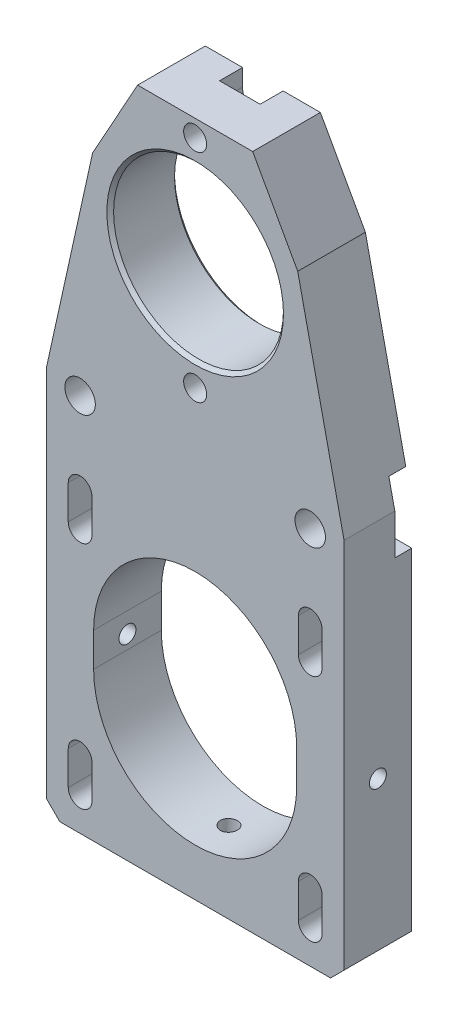
from build123d import *

# Parameters (mm, degrees)
SKETCH1_W                                            = 44
SKETCH1_H                                            = 100
BOSS_EXTRUDE1_DEPTH                                  = 10
SKETCH2_R                                            = 12.55
CUT_EXTRUDE1_DEPTH                                   = 56.533773508
CUT_EXTRUDE3_DEPTH                                   = 56.533773508
CUT_EXTRUDE12_DEPTH                                  = 4.6
LPATTERN1_COUNT                                      = 2
LPATTERN1_PITCH                                      = 34
LPATTERN1_COUNT_DIR2                                 = 2
LPATTERN1_PITCH_DIR2                                 = 34
CHAMFER1_SIZE                                        = 2
CUT_EXTRUDE10_DEPTH                                  = 56.533773508
CUT_EXTRUDE11_DEPTH                                  = 10
M3_TAPPED_HOLE3_D                                    = 2.5
SKETCH27_W                                           = 62.376043996
SKETCH27_H                                           = 10
CUT_EXTRUDE13_DEPTH                                  = 2.5
SKETCH6_R                                            = 2.25
CUT_EXTRUDE5_DEPTH                                   = 10
CHAMFER2_SIZE                                        = 0.5
HOLE_SIZE_PER_SOCKET_HEAD_CAP_SCREW_TYPE_D           = 3.4
HOLE_SIZE_PER_SOCKET_HEAD_CAP_SCREW_TYPE_CBORE_D     = 6
HOLE_SIZE_PER_SOCKET_HEAD_CAP_SCREW_TYPE_CBORE_DEPTH = 3.4
CUT_EXTRUDE14_DEPTH                                  = 3.4
M3_TAPPED_HOLE5_D                                    = 2.5
M3_TAPPED_HOLE5_DEPTH                                = 7.5
M3_TAPPED_HOLE5_TIP                                  = 0.751075774


with BuildPart() as part:
    # Sketch1 → Boss-Extrude1 (new body)
    with BuildSketch(Plane.XY):
        Rectangle(SKETCH1_W, SKETCH1_H)
    extrude(amount=BOSS_EXTRUDE1_DEPTH)

    # Sketch2 → Cut-Extrude1 (cut, through all)
    with BuildSketch(Plane.XY.offset(10)):
        with Locations((0, 31.5)):
            Circle(SKETCH2_R)
        with BuildLine():
            Line((-15, -28), (-15, -23))
            ThreePointArc((-15, -23), (0, -8), (15, -23))
            Line((15, -23), (15, -28))
            ThreePointArc((15, -28), (0, -43), (-15, -28))
        make_face()
    extrude(amount=-CUT_EXTRUDE1_DEPTH, mode=Mode.SUBTRACT)

    # Sketch4 → Cut-Extrude3 (cut, through all)
    with BuildSketch(Plane.XY.offset(10)):
        with BuildLine():
            Line((-15.25, -6), (-15.25, -11))
            ThreePointArc((-15.25, -11), (-17, -12.75), (-18.75, -11))
            Line((-18.75, -11), (-18.75, -6))
            ThreePointArc((-18.75, -6), (-17, -4.25), (-15.25, -6))
        make_face()
        with BuildLine():
            Line((18.75, -6), (18.75, -11))
            ThreePointArc((18.75, -11), (17, -12.75), (15.25, -11))
            Line((15.25, -11), (15.25, -6))
            ThreePointArc((15.25, -6), (17, -4.25), (18.75, -6))
        make_face()
        with BuildLine():
            Line((18.75, -40), (18.75, -45))
            ThreePointArc((18.75, -45), (17, -46.75), (15.25, -45))
            Line((15.25, -45), (15.25, -40))
            ThreePointArc((15.25, -40), (17, -38.25), (18.75, -40))
        make_face()
        with BuildLine():
            Line((-15.25, -40), (-15.25, -45))
            ThreePointArc((-15.25, -45), (-17, -46.75), (-18.75, -45))
            Line((-18.75, -45), (-18.75, -40))
            ThreePointArc((-18.75, -40), (-17, -38.25), (-15.25, -40))
        make_face()
    extrude(amount=-CUT_EXTRUDE3_DEPTH, mode=Mode.SUBTRACT)

    # Sketch20 → Cut-Extrude12 (cut)
    with BuildSketch(Plane(origin=(0, 0, 0), x_dir=(-1, 0, 0), z_dir=(0, 0, -1))):
        with BuildLine():
            Line((19.9, -6), (19.9, -11))
            ThreePointArc((19.9, -11), (17, -13.9), (14.1, -11))
            Line((14.1, -11), (14.1, -6))
            ThreePointArc((14.1, -6), (17, -3.1), (19.9, -6))
        make_face()
    cut_extrude12 = extrude(amount=-CUT_EXTRUDE12_DEPTH, mode=Mode.SUBTRACT)

    # LPattern1: Cut-Extrude12 2 × 2
    with Locations(*[(j * LPATTERN1_PITCH_DIR2, -i * LPATTERN1_PITCH, 0) for i in range(LPATTERN1_COUNT) for j in range(LPATTERN1_COUNT_DIR2) if (i, j) != (0, 0)]):
        add(cut_extrude12, mode=Mode.SUBTRACT)

    # Chamfer1
    chamfer1_edges = [part.edges().sort_by_distance(p)[0] for p in [
        (22, -50, 5),
        (-22, -50, 5),
    ]]
    chamfer(chamfer1_edges, length=CHAMFER1_SIZE)

    # Sketch15 → Cut-Extrude10 (cut, through all)
    with BuildSketch(Plane.XY.offset(10)):
        Polygon((22, 7), (12.5, 50), (22, 50), align=None)
        Polygon((-12.5, 50), (-22, 7), (-22, 50), align=None)
    extrude(amount=-CUT_EXTRUDE10_DEPTH, mode=Mode.SUBTRACT)

    # Sketch16 → Cut-Extrude11 (cut)
    with BuildSketch(Plane.XY.offset(10)):
        Polygon((-12.5, 50), (-8.5, 50), (-15.151162791, 38), align=None)
    cut_extrude11 = extrude(amount=-CUT_EXTRUDE11_DEPTH, mode=Mode.SUBTRACT)

    # Mirror2: Cut-Extrude11 across plane
    add(cut_extrude11.mirror(Plane(origin=(0, 0, 0), x_dir=(0, 0, 1), z_dir=(1, 0, 0))), mode=Mode.SUBTRACT)

    # M3 Tapped Hole3 (through all)
    with Locations(Plane.XY.offset(10)):
        with Locations((0, 47.5), (0, 15.5)):
            Hole(M3_TAPPED_HOLE3_D / 2)

    # Sketch27 → Cut-Extrude13 (cut)
    with BuildSketch(Plane(origin=(0, 0, 0), x_dir=(-1, 0, 0), z_dir=(0, 0, -1))):
        with Locations((-1.474712029, 6)):
            Rectangle(SKETCH27_W, SKETCH27_H)
    extrude(amount=-CUT_EXTRUDE13_DEPTH, mode=Mode.SUBTRACT)

    # Sketch6 → Cut-Extrude5 (cut)
    with BuildSketch(Plane.XY.offset(10)):
        with Locations((-17, 6)):
            Circle(SKETCH6_R)
        with Locations((17, 6)):
            Circle(SKETCH6_R)
    extrude(amount=-CUT_EXTRUDE5_DEPTH, mode=Mode.SUBTRACT)

    # Chamfer2
    chamfer2_edges = [part.edges().sort_by_distance(p)[0] for p in [
        (-12.55, 31.5, 0),
        (-12.55, 31.5, 10),
    ]]
    chamfer(chamfer2_edges, length=CHAMFER2_SIZE)

    # Hole size per socket head cap screw type 1 (through all)
    with Locations(Plane(origin=(0, 0, 0), x_dir=(-1, 0, 0), z_dir=(0, 0, -1))):
        with Locations((0, 47.5), (0, 15.5)):
            CounterBoreHole(HOLE_SIZE_PER_SOCKET_HEAD_CAP_SCREW_TYPE_D / 2, HOLE_SIZE_PER_SOCKET_HEAD_CAP_SCREW_TYPE_CBORE_D / 2, HOLE_SIZE_PER_SOCKET_HEAD_CAP_SCREW_TYPE_CBORE_DEPTH)

    # Sketch30 → Cut-Extrude14 (cut)
    with BuildSketch(Plane(origin=(0, 0, 0), x_dir=(-1, 0, 0), z_dir=(0, 0, -1))):
        with BuildLine():
            Line((-3, 47.5), (-3, 54.060013121))
            ThreePointArc((-3, 54.060013121), (0, 57.060013121), (3, 54.060013121))
            Line((3, 54.060013121), (3, 47.5))
            ThreePointArc((3, 47.5), (0, 44.5), (-3, 47.5))
        make_face()
    extrude(amount=-CUT_EXTRUDE14_DEPTH, mode=Mode.SUBTRACT)

    # Sketch31 → M3 Tapped Hole4 (revolve, cut)
    with BuildSketch(Plane(origin=(22, -26, 5), x_dir=(0, 0, -1), z_dir=(0, 1, 0))):
        Polygon((0, 0), (0, 8.251075774), (1.25, 7.5), (1.25, 0), align=None)
    m3_tapped_hole4 = revolve(axis=Axis((28.35, -26, 5), (-1, 0, 0)), mode=Mode.SUBTRACT)

    # Mirror3: M3 Tapped Hole4 across plane
    add(m3_tapped_hole4.mirror(Plane(origin=(0, 0, 0), x_dir=(0, 0, 1), z_dir=(1, 0, 0))), mode=Mode.SUBTRACT)

    # M3 Tapped Hole5
    with Locations(Plane(origin=(0, -50, 0), x_dir=(-1, 0, 0), z_dir=(0, -1, 0))):
        with Locations((0, -5)):
            Hole(M3_TAPPED_HOLE5_D / 2, depth=M3_TAPPED_HOLE5_DEPTH)
            with Locations((0, 0, -(M3_TAPPED_HOLE5_DEPTH + M3_TAPPED_HOLE5_TIP / 2))):  # 118° drill point
                Cone(0, M3_TAPPED_HOLE5_D / 2, M3_TAPPED_HOLE5_TIP, mode=Mode.SUBTRACT)


solid = part.part
